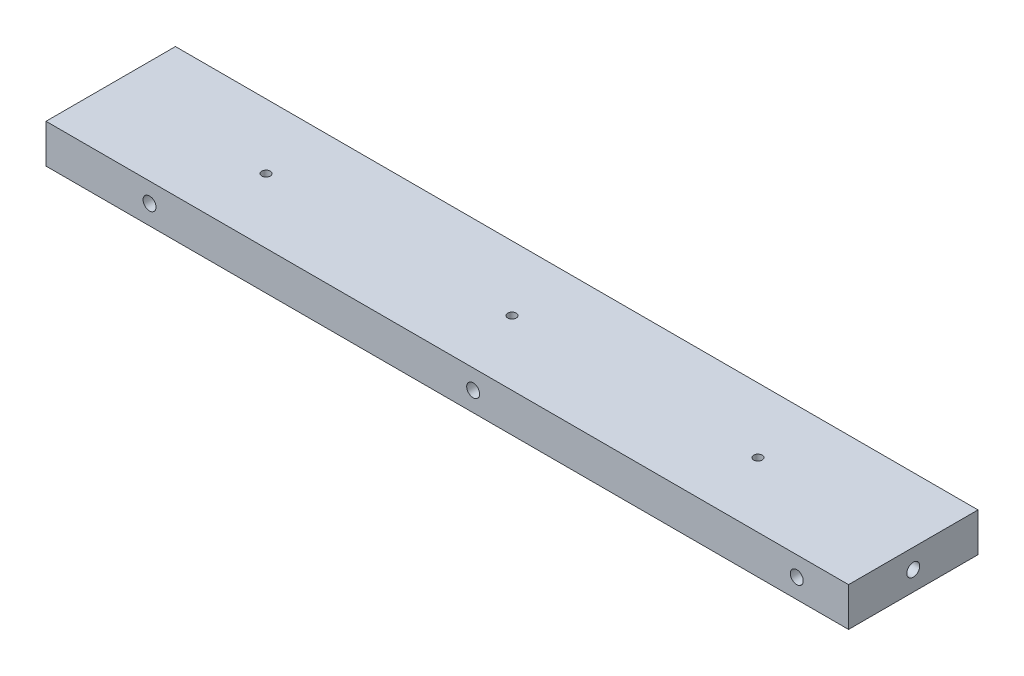
SolidWorks part; units mm, degrees
material "6061"
ref_plane "前视基准面" through (0, 0, 0) normal (0, 0, 1) x (1, 0, 0)
ref_plane "上视基准面" through (0, 0, 0) normal (0, 1, 0) x (1, 0, 0)
ref_plane "右视基准面" through (0, 0, 0) normal (1, 0, 0) x (0, 0, -1)
sketch "草图1" plane through (0, 0, 0) normal (0, 1, 0) x (1, 0, 0)
  line L1 (155, -25) -> (-155, -25)
  line L2 (155, -25) -> (155, 25)
  line L3 (155, 25) -> (-155, 25)
  line L4 (-155, -25) -> (-155, 25)
  line L5 (155, -25) -> (-155, 25) construction
  line L6 (155, 25) -> (-155, -25) construction
  point P0 (0, 0)
  dimension "D1" = 310
  dimension "D2" = 50
extrude "凸台-拉伸1" add sketch "草图1" along normal mid plane 15
hole_wizard "M6 螺纹孔1" positions "草图2" profile "草图3" tap size "M6" standard "ISO"
sketch "草图2" plane through (0, 0, 25) normal (0, 0, 1) x (1, 0, 0)
  point P0 (-115, 0)
  point P3 (10, 0)
  point P6 (135, 0)
cosmetic thread "孔螺蚊线1" parameters "D1"=12, "D2"=6
cosmetic thread "孔螺蚊线2" parameters "D1"=12, "D2"=6
cosmetic thread "孔螺蚊线3" parameters "D1"=12, "D2"=6
sketch "草图3" plane through (-115, 0, 25) normal (1, 0, 0) x (0, -1, 0)
  line L0 (0, 0) -> (0, 18.5022)
  line L1 (0, 18.5022) -> (2.5, 17)
  line L2 (2.5, 17) -> (2.5, 0)
  line L5 (2.5, 0) -> (0, 0)
  line L10 (0, 18.5022) -> (-2.5, 17) construction
  line L11 (0, -6.35) -> (0, 107.95) construction
  dimension "螺纹孔钻头直径" = 5
  dimension "螺纹孔钻头深度" = 17
  dimension "导头角度" = 118
hole_wizard "M6 螺纹孔2" positions "草图4" profile "草图6" tap size "M6" standard "ISO"
sketch "草图4" plane through (155, 0, 0) normal (1, 0, 0) x (0, 0, -1)
  point P0 (0, 0)
sketch "草图6" plane through (155, 0, 0) normal (0, 1, 0) x (0, 0, -1)
  line L0 (0, 0) -> (0, 18.5022)
  line L1 (0, 18.5022) -> (2.5, 17)
  line L2 (2.5, 17) -> (2.5, 0)
  line L5 (2.5, 0) -> (0, 0)
  line L10 (0, 18.5022) -> (-2.5, 17) construction
  line L11 (0, -6.35) -> (0, 107.95) construction
  dimension "螺纹孔钻头直径" = 5
  dimension "螺纹孔钻头深度" = 17
  dimension "导头角度" = 118
cosmetic thread "孔螺蚊线4" parameters "D1"=12, "D2"=6
hole_wizard "M6 螺纹孔3" positions "草图7" profile "草图8" tap size "M6" standard "ISO"
sketch "草图7" plane through (-155, 0, 0) normal (-1, 0, 0) x (0, 0, 1)
  point P0 (0, 0)
sketch "草图8" plane through (-155, 0, 0) normal (0, 1, 0) x (0, 0, 1)
  line L0 (0, 0) -> (0, 18.5022)
  line L1 (0, 18.5022) -> (2.5, 17)
  line L2 (2.5, 17) -> (2.5, 0)
  line L5 (2.5, 0) -> (0, 0)
  line L10 (0, 18.5022) -> (-2.5, 17) construction
  line L11 (0, -6.35) -> (0, 107.95) construction
  dimension "螺纹孔钻头直径" = 5
  dimension "螺纹孔钻头深度" = 17
  dimension "导头角度" = 118
cosmetic thread "孔螺蚊线5" parameters "D1"=12, "D2"=6
hole_wizard "M4 螺纹孔1" positions "草图9" profile "草图10" tap size "M4" standard "GB" end condition through all
sketch "草图9" plane through (0, 7.5, 0) normal (0, 1, 0) x (1, 0, 0)
  line L0 (-155, 0) -> (155, 0) construction
  line L1 (-155, 25) -> (-155, -25) construction
  line L2 (155, -25) -> (155, 25) construction
  point P0 (-95, 0)
  point P2 (0, 0)
  point P5 (95, 0)
  dimension "D1" = 60
  dimension "D2" = 190
sketch "草图10" plane through (-95, 7.5, 0) normal (1, 0, 0) x (0, 0, 1)
  line L0 (0, 0) -> (0, 15)
  line L1 (0, 15) -> (1.65, 15)
  line L2 (1.65, 15) -> (1.65, 0)
  line L5 (1.65, 0) -> (0, 0)
  line L11 (0, -6.35) -> (0, 107.95) construction
  dimension "通孔螺纹孔钻头直径" = 3.3
  dimension "通孔螺纹孔钻头深度" = 15
cosmetic thread "孔螺蚊线6" parameters "D2"=4
cosmetic thread "孔螺蚊线7" parameters "D2"=4
cosmetic thread "孔螺蚊线8" parameters "D2"=4
